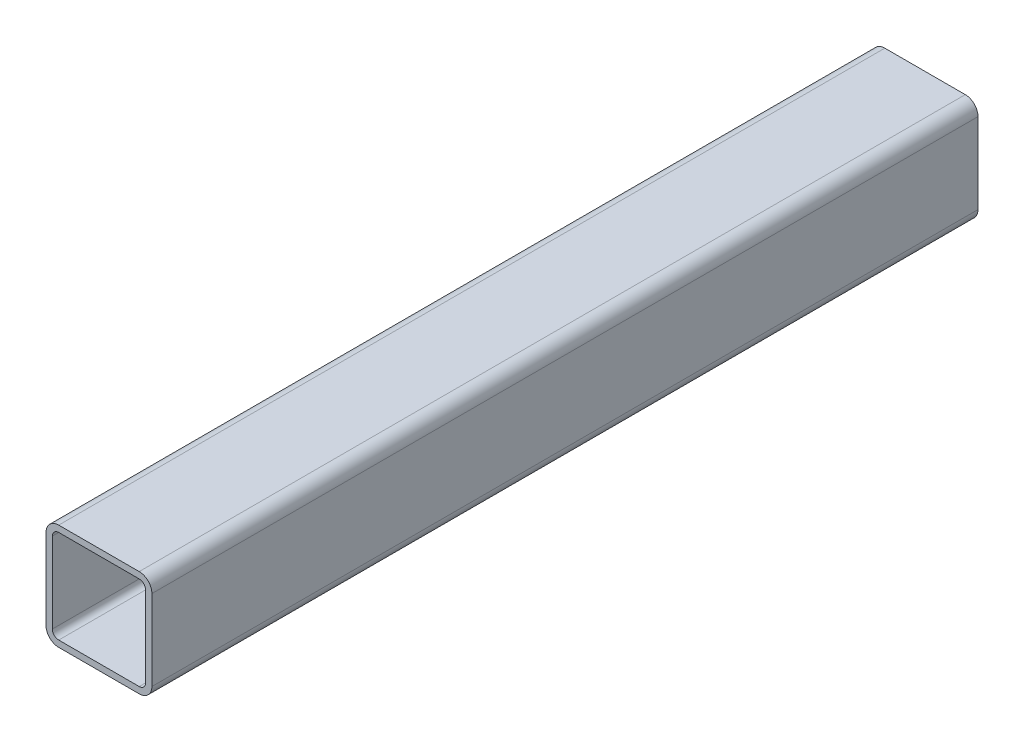
SolidWorks part; units mm, degrees
material "Q235B"
ref_plane "前视基准面" through (0, 0, 0) normal (0, 0, 1) x (1, 0, 0)
ref_plane "上视基准面" through (0, 0, 0) normal (0, 1, 0) x (1, 0, 0)
ref_plane "右视基准面" through (0, 0, 0) normal (1, 0, 0) x (0, 0, -1)
other "Configuration Table"
sketch "草图1" plane through (0, 0, 0) normal (1, 0, 0) x (0, 0, -1)
  line L0 (-195, 0) -> (195, 0)
other "Gb／6728-1986方形空心型钢 050 X 50 X 3(1)"
ref_plane "基准面1" through (0, 0, 195) normal (0, 0, -1) x (0, 1, 0)
sketch "Sketch1" plane through (0, 0, 195) normal (0, 0, -1) x (0, 1, 0)
  line L0 (-19, -22) -> (19, -22)
  line L1 (-22, -19) -> (-22, 19)
  line L2 (19, 22) -> (-19, 22)
  line L3 (22, 19) -> (22, -19)
  line L4 (-19, -25) -> (19, -25)
  line L5 (-25, -19) -> (-25, 19)
  line L6 (19, 25) -> (-19, 25)
  line L7 (25, 19) -> (25, -19)
  arc A0 (25, 19) -> (19, 25) centre (19, 19) ccw
  arc A1 (19, -25) -> (25, -19) centre (19, -19) ccw
  arc A2 (-25, -19) -> (-19, -25) centre (-19, -19) ccw
  arc A3 (-19, 25) -> (-25, 19) centre (-19, 19) ccw
  arc A4 (-19, 22) -> (-22, 19) centre (-19, 19) ccw
  arc A5 (22, 19) -> (19, 22) centre (19, 19) ccw
  arc A6 (19, -22) -> (22, -19) centre (19, -19) ccw
  arc A7 (-22, -19) -> (-19, -22) centre (-19, -19) ccw
  point P0 (-25, 0)
  point P1 (25, 0)
  point P2 (0, 25)
  point P3 (0, -25)
  point P4 (0, 0)
  point P5 (-25, -25)
  point P6 (25, -25)
  point P7 (25, 25)
  point P8 (-25, 25)
  point P33 (0, 0)
  dimension "D1" = 6
  dimension "Thickness" = 3
  dimension "V_leg" = 50
equation "\"D2@草图1\"=\"D1@草图1\"/2"
